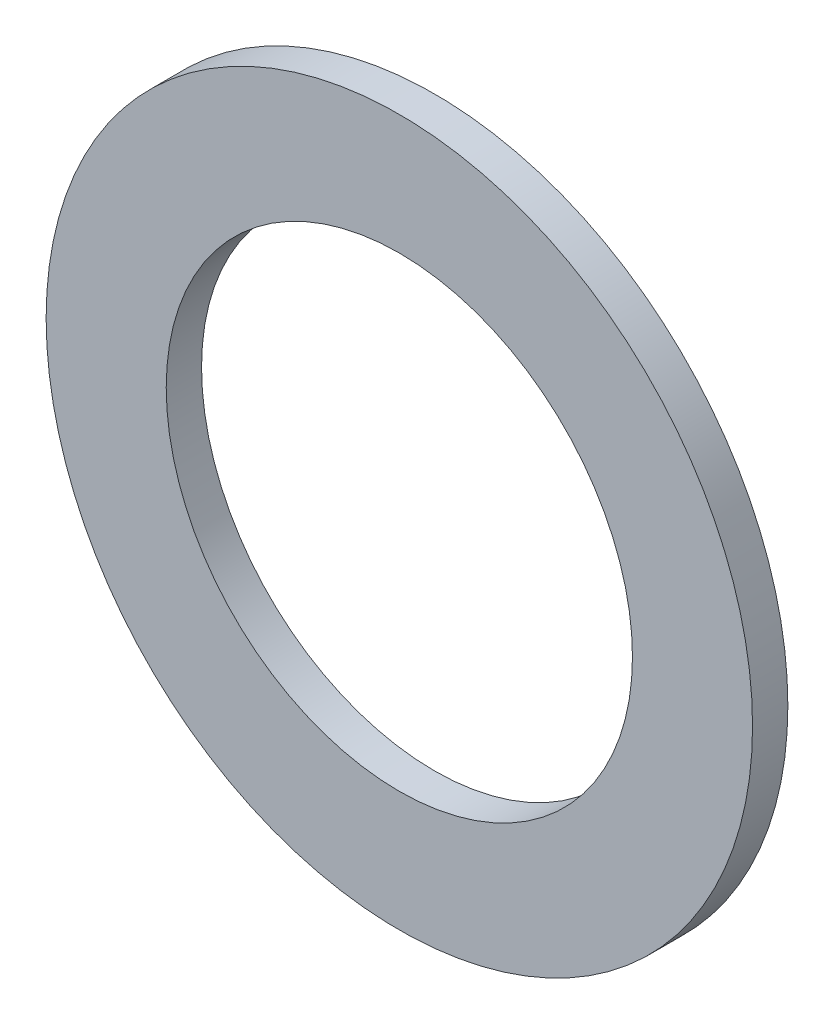
SolidWorks part; units mm, degrees
material "普通碳钢"
ref_plane "前视" through (0, 0, 0) normal (0, 0, 1) x (1, 0, 0)
ref_plane "上视" through (0, 0, 0) normal (0, 1, 0) x (1, 0, 0)
ref_plane "右视" through (0, 0, 0) normal (1, 0, 0) x (0, 0, -1)
sketch "草图1" plane through (0, 0, 0) normal (0, 0, 1) x (1, 0, 0)
  line L0 (-97.43, 0) -> (95.7164, 0) construction
  line L1 (0, 69.8901) -> (0, -65.7285) construction
  circle A0 centre (0, 0) radius 50
  circle A1 centre (0, 0) radius 33
  dimension "D1" = 66
  dimension "D2" = 100
extrude "凸台-拉伸1" add sketch "草图1" along normal blind 5
